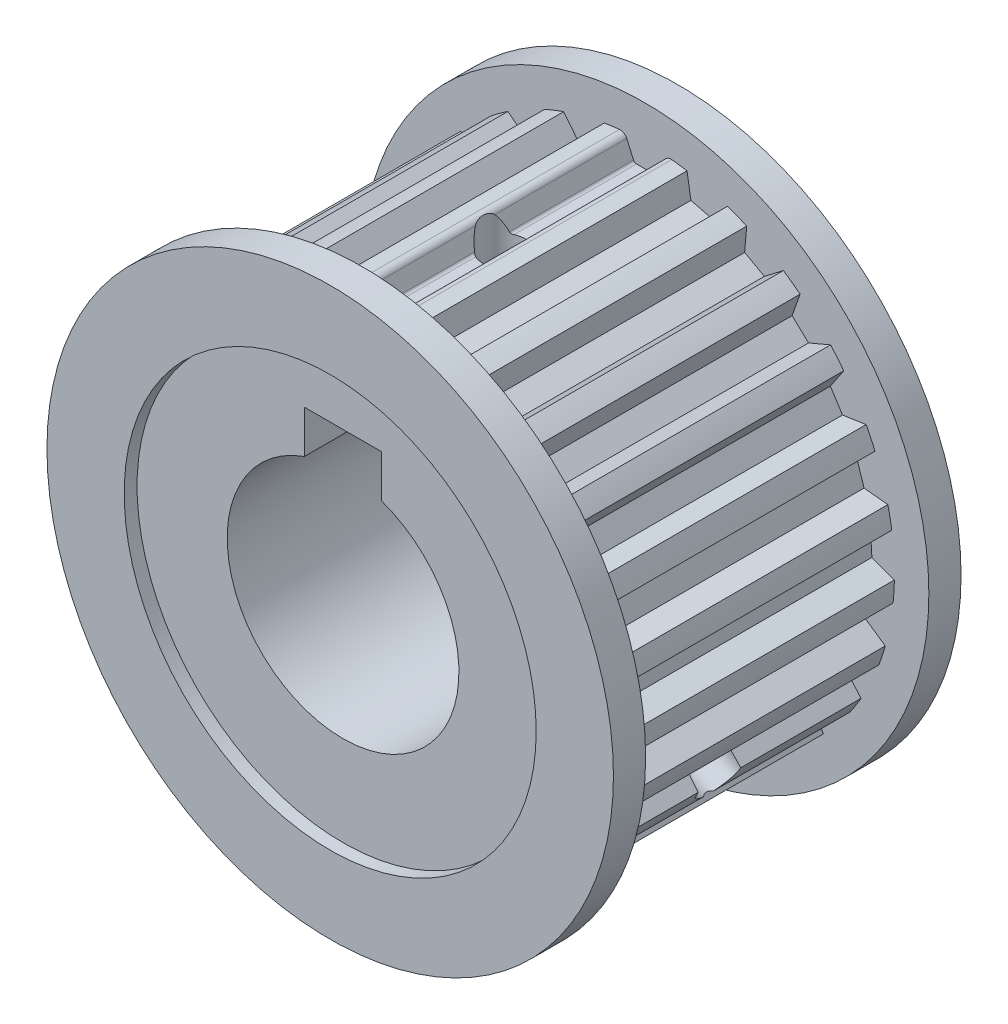
from build123d import *

# Parameters (mm, degrees)
SKETCH_1_R               = 19.325
EXTRUDE_1_DEPTH          = 13.5
CUT_EXTRUDE_1_DEPTH      = 13.5
FILLET_3_R               = 0.55
FILLET_4_R               = 0.25
PATTERN_CIRCULAR_2_COUNT = 25
SKETCH_3_R               = 22
EXTRUDE_2_DEPTH          = 2.5
SKETCH_4_R               = 16
CUT_EXTRUDE_2_DEPTH      = 1
CUT_EXTRUDE_3_DEPTH      = 13.5
SKETCH_6_W               = 1.65
SKETCH_6_H               = 30.052558883
PATTERN_CIRCULAR_3_COUNT = 2
PATTERN_CIRCULAR_3_ANGLE = 120


with BuildPart() as part:
    # 草图1 → 凸台-拉伸1 (new, symmetric)
    with BuildSketch(Plane.XY):
        Circle(SKETCH_1_R)
    extrude(amount=EXTRUDE_1_DEPTH, both=True)

    # 草图2 → 切除-拉伸1 (cut, symmetric)
    with BuildSketch(Plane.XY):
        with BuildLine():
            Line((-0.875, 17.555), (0.875, 17.555))
            Line((0.875, 17.555), (1.625, 19.256557325))
            ThreePointArc((1.625, 19.256557325), (0, 19.325), (-1.625, 19.256557325))
            Line((-1.625, 19.256557325), (-0.875, 17.555))
        make_face()
    cut_extrude_1 = extrude(amount=CUT_EXTRUDE_1_DEPTH, both=True, mode=Mode.SUBTRACT)

    # 圆角3
    fillet_3_edges = [part.edges().sort_by_distance(p)[0] for p in [
        (-1.625, 19.256557325, 0),
        (1.625, 19.256557325, 0),
    ]]
    fillet(fillet_3_edges, radius=FILLET_3_R)

    # 圆角4
    fillet_4_edges = [part.edges().sort_by_distance(p)[0] for p in [
        (-0.875, 17.555, 0),
        (0.875, 17.555, 0),
    ]]
    fillet(fillet_4_edges, radius=FILLET_4_R)

    # 阵列(圆周)2: 切除-拉伸1 ×25 about axis
    pattern_circular_2_axis = Axis((0, 0, 0), (0, 0, 1))
    for i in range(1, PATTERN_CIRCULAR_2_COUNT):
        add(cut_extrude_1.rotate(pattern_circular_2_axis, i * 360 / PATTERN_CIRCULAR_2_COUNT), mode=Mode.SUBTRACT)

    # 草图3 → 凸台-拉伸2 (add)
    with BuildSketch(Plane.XY.offset(13.5)):
        Circle(SKETCH_3_R)
    extrude_2 = extrude(amount=-EXTRUDE_2_DEPTH)

    # 镜向1: 凸台-拉伸2 across plane
    add(extrude_2.mirror(Plane.XY))

    # 草图4 → 切除-拉伸2 (cut)
    with BuildSketch(Plane.XY.offset(13.5)):
        Circle(SKETCH_4_R)
    cut_extrude_2 = extrude(amount=-CUT_EXTRUDE_2_DEPTH, mode=Mode.SUBTRACT)

    # 镜向2: 切除-拉伸2 across plane
    add(cut_extrude_2.mirror(Plane.XY), mode=Mode.SUBTRACT)

    # 草图5 → 切除-拉伸3 (cut, symmetric)
    with BuildSketch(Plane.XY):
        with BuildLine():
            Line((-3, 11.8), (3, 11.8))
            Line((3, 11.8), (3, 8.485281374))
            ThreePointArc((3, 8.485281374), (0, -9), (-3, 8.485281374))
            Line((-3, 8.485281374), (-3, 11.8))
        make_face()
    extrude(amount=CUT_EXTRUDE_3_DEPTH, both=True, mode=Mode.SUBTRACT)

    # 草图6 → M4 螺纹孔1 (revolve, cut)
    with BuildSketch(Plane(origin=(0, 0, 0), x_dir=(0, 0, -1), z_dir=(1, 0, 0))):
        with Locations((0.825, 15.026279442)):
            Rectangle(SKETCH_6_W, SKETCH_6_H)
    hole_wizard_m4_1 = revolve(axis=Axis((0, -6.35, 0), (0, 1, 0)), mode=Mode.SUBTRACT)

    # 阵列(圆周)3: M4 螺纹孔1 ×2 about axis
    pattern_circular_3_axis = Axis((0, 0, 13.5), (0, 0, -1))
    for i in range(1, PATTERN_CIRCULAR_3_COUNT):
        add(hole_wizard_m4_1.rotate(pattern_circular_3_axis, i * PATTERN_CIRCULAR_3_ANGLE / (PATTERN_CIRCULAR_3_COUNT - 1)), mode=Mode.SUBTRACT)


solid = part.part
